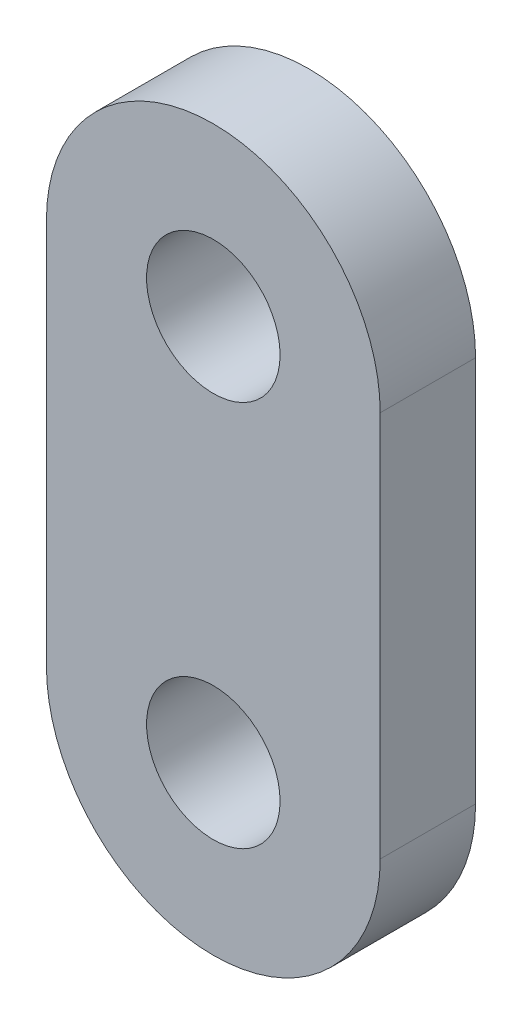
SolidWorks part; units mm, degrees
material "AISI 1045 钢，冷拔"
ref_plane "Front Plane" through (0, 0, 0) normal (0, 0, 1) x (1, 0, 0)
ref_plane "Top Plane" through (0, 0, 0) normal (0, 1, 0) x (1, 0, 0)
ref_plane "Right Plane" through (0, 0, 0) normal (1, 0, 0) x (0, 0, -1)
sketch "Sketch1" plane through (0, 0, 0) normal (0, 0, 1) x (1, 0, 0)
  line L0 (-8.75, 0) -> (-8.75, -20.26)
  line L1 (0, 13.2547) -> (0, -33.3576) construction
  line L2 (8.75, 0) -> (8.75, -20.26)
  circle A0 centre (0, 0) radius 3.5
  circle A1 centre (0, -20.26) radius 3.5
  arc A2 (8.75, 0) -> (-8.75, 0) centre (0, 0) ccw
  arc A3 (-8.75, -20.26) -> (8.75, -20.26) centre (0, -20.26) ccw
  dimension "D1" = 7
  dimension "D2" = 7
  dimension "D3" = 20.26
  dimension "D4" = 17.5
  dimension "D5" = 17.5
extrude "Boss-Extrude1" add sketch "Sketch1" along normal blind 5
